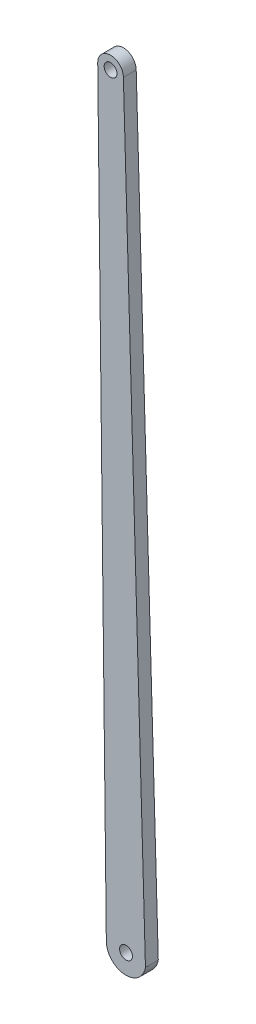
from build123d import *

# Parameters (mm, degrees)
SKETCH3_R           = 5
BOSS_EXTRUDE1_DEPTH = 10


with BuildPart() as part:
    # Sketch3 → Boss-Extrude1 (new body)
    # profile 1 of 6: a face of its own
    with BuildSketch(Plane.XY):
        with BuildLine():
            Line((27.39481576, 680.560432475), (27.230443202, 686.220183409))
            Line((27.230443202, 686.220183409), (13.205751534, 1169.124769421))
            ThreePointArc((13.205751534, 1169.124769421), (2.770474558, 1164.302567957), (-8.590118071, 1166.059146344))
            Line((-8.590118071, 1166.059146344), (-3.095663833, 682.778262513))
            ThreePointArc((-3.095663833, 682.778262513), (11.13008439, 667.653491235), (27.39481576, 680.560432475))
        make_face()
        with Locations((12.242921242, 682.952647962)):
            Circle(SKETCH3_R, mode=Mode.SUBTRACT)
    # profile 2 of 6: a face of its own
    with BuildSketch(Plane.XY):
        with BuildLine():
            ThreePointArc((-8.590118071, 1166.059146344), (2.770474558, 1164.302567957), (13.205751534, 1169.124769421))
            Line((13.205751534, 1169.124769421), (10.388282273, 1266.137157238))
            ThreePointArc((10.388282273, 1266.137157238), (5.346882565, 1267.310168836), (0.186416397, 1267.711735959))
            ThreePointArc((0.186416397, 1267.711735959), (-4.824372475, 1267.355069011), (-9.729431527, 1266.270812525))
            Line((-9.729431527, 1266.270812525), (-8.590118071, 1166.059146344))
        make_face()
        with Locations((0, 1184)):
            Circle(SKETCH3_R, mode=Mode.SUBTRACT)
    # profile 3 of 6: a face of its own
    with BuildSketch(Plane.XY):
        with BuildLine():
            ThreePointArc((0.186416397, 1267.711735959), (5.346882565, 1267.310168836), (10.388282273, 1266.137157238))
            Line((10.388282273, 1266.137157238), (10.197341299, 1272.711724024))
            ThreePointArc((10.197341299, 1272.711724024), (9.983454072, 1274.768905783), (9.35094194, 1276.738086563))
            ThreePointArc((9.35094194, 1276.738086563), (4.804919365, 1277.462611062), (0.208267791, 1277.711712085))
            ThreePointArc((0.208267791, 1277.711712085), (3.736736195, 1276.243392718), (5.197341299, 1272.711724024))
            ThreePointArc((5.197341299, 1272.711724024), (3.729010557, 1269.172329689), (0.186416397, 1267.711735959))
        make_face()
    # profile 4 of 6: a face of its own
    with BuildSketch(Plane.XY):
        with BuildLine():
            ThreePointArc((0.208267791, 1277.711712085), (4.804919365, 1277.462611062), (9.35094194, 1276.738086563))
            ThreePointArc((9.35094194, 1276.738086563), (0.219193138, 1282.711700148), (-8.938575282, 1276.778052618))
            ThreePointArc((-8.938575282, 1276.778052618), (-4.38942912, 1277.482702512), (0.208267791, 1277.711712085))
        make_face()
    # profile 5 of 6: a face of its own
    with BuildSketch(Plane.XY):
        with BuildLine():
            ThreePointArc((-9.729431527, 1266.270812525), (-4.824372475, 1267.355069011), (0.186416397, 1267.711735959))
            ThreePointArc((0.186416397, 1267.711735959), (-4.802646764, 1272.722649721), (0.208267791, 1277.711712085))
            ThreePointArc((0.208267791, 1277.711712085), (-4.38942912, 1277.482702512), (-8.938575282, 1276.778052618))
            ThreePointArc((-8.938575282, 1276.778052618), (-9.584252789, 1274.790285328), (-9.802658701, 1272.711724024))
            Line((-9.802658701, 1272.711724024), (-9.80007392, 1272.484372008))
            Line((-9.80007392, 1272.484372008), (-9.729431527, 1266.270812525))
        make_face()
    # profile 6 of 6: a face of its own
    with BuildSketch(Plane.XY):
        with Locations((0, 1184)):
            Circle(SKETCH3_R)
    extrude(amount=BOSS_EXTRUDE1_DEPTH)


solid = part.part
